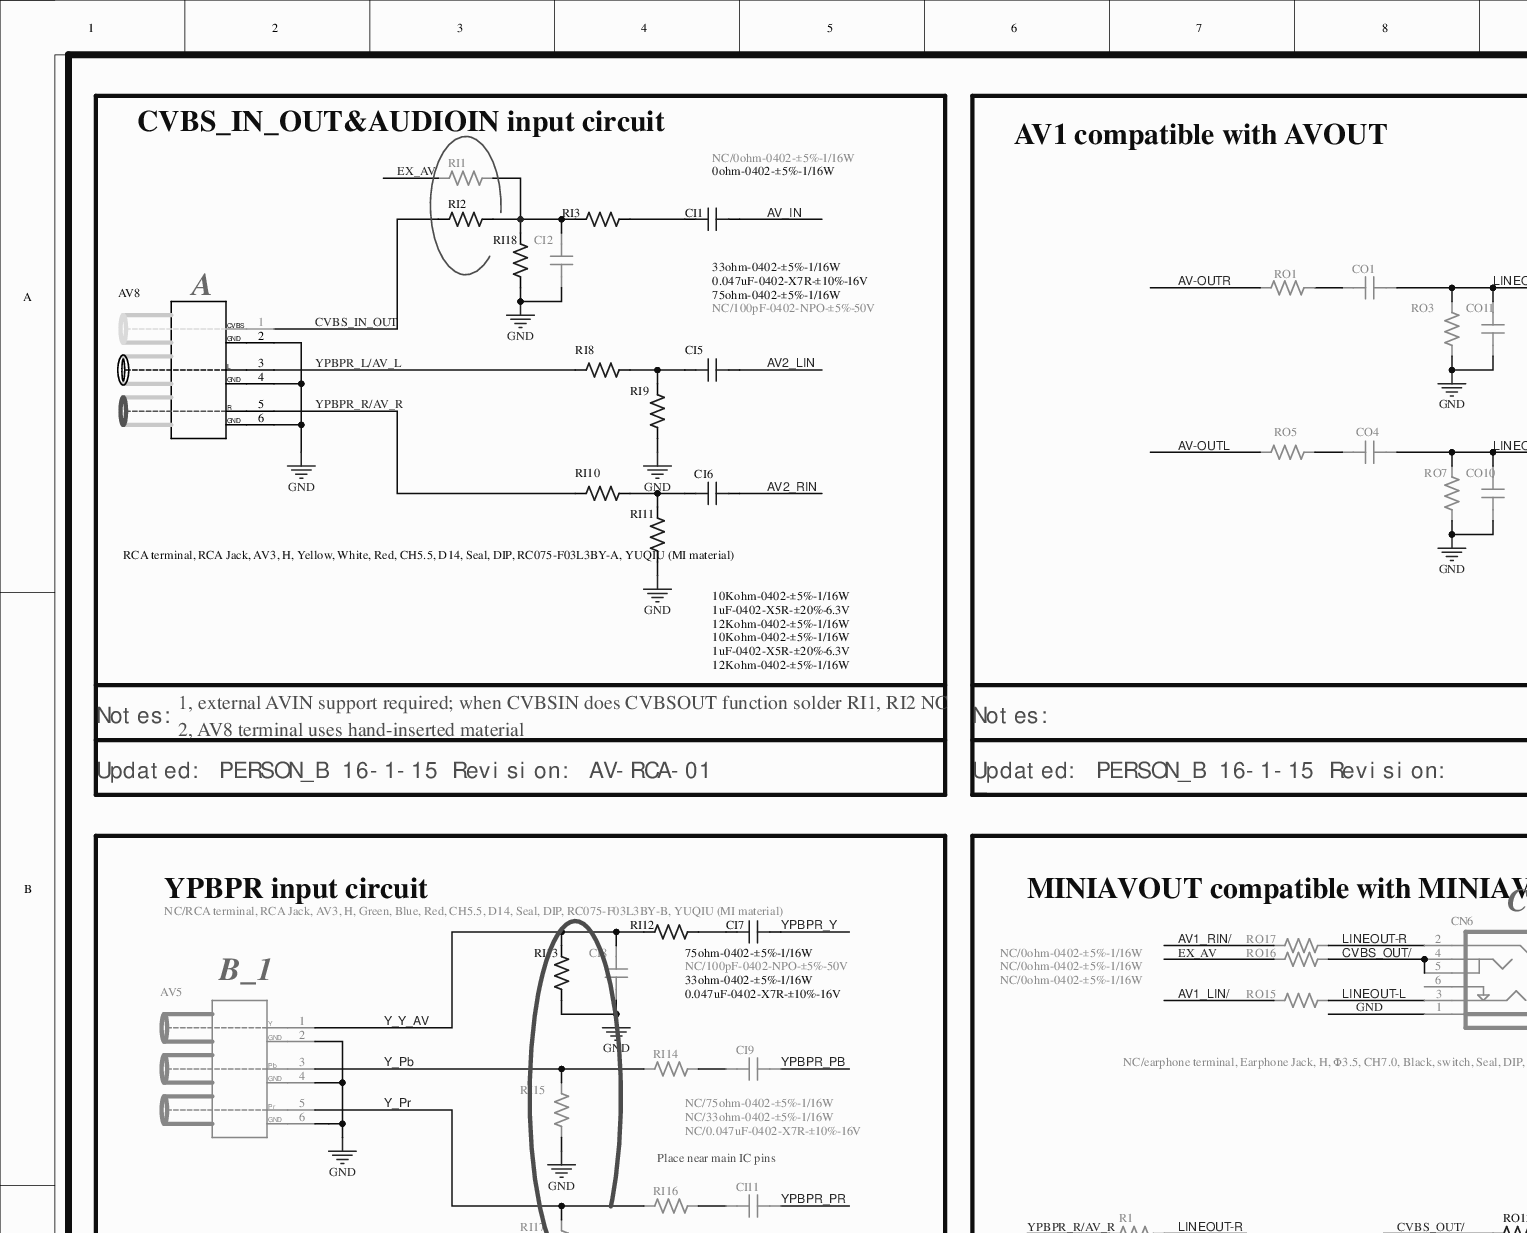
[diagram p0: MISC84277-9.SchDoc, top left]
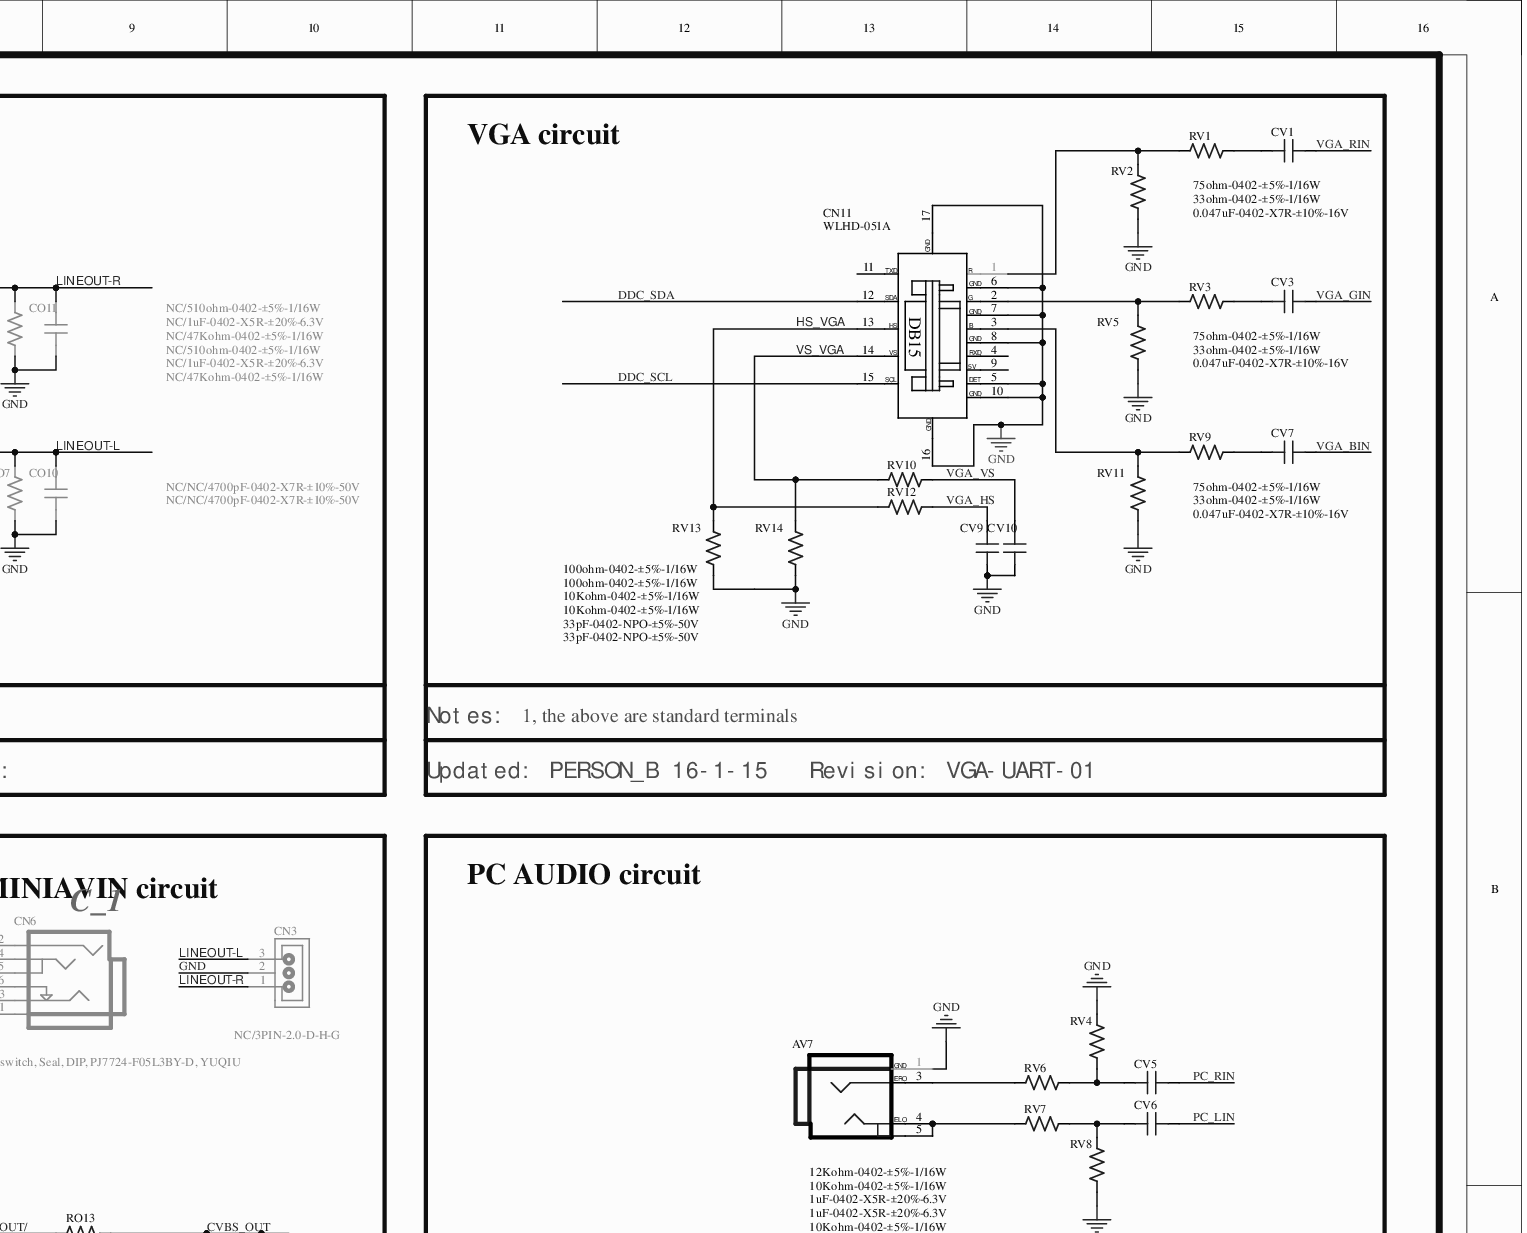
[diagram p1: MISC84277-9.SchDoc, top right]
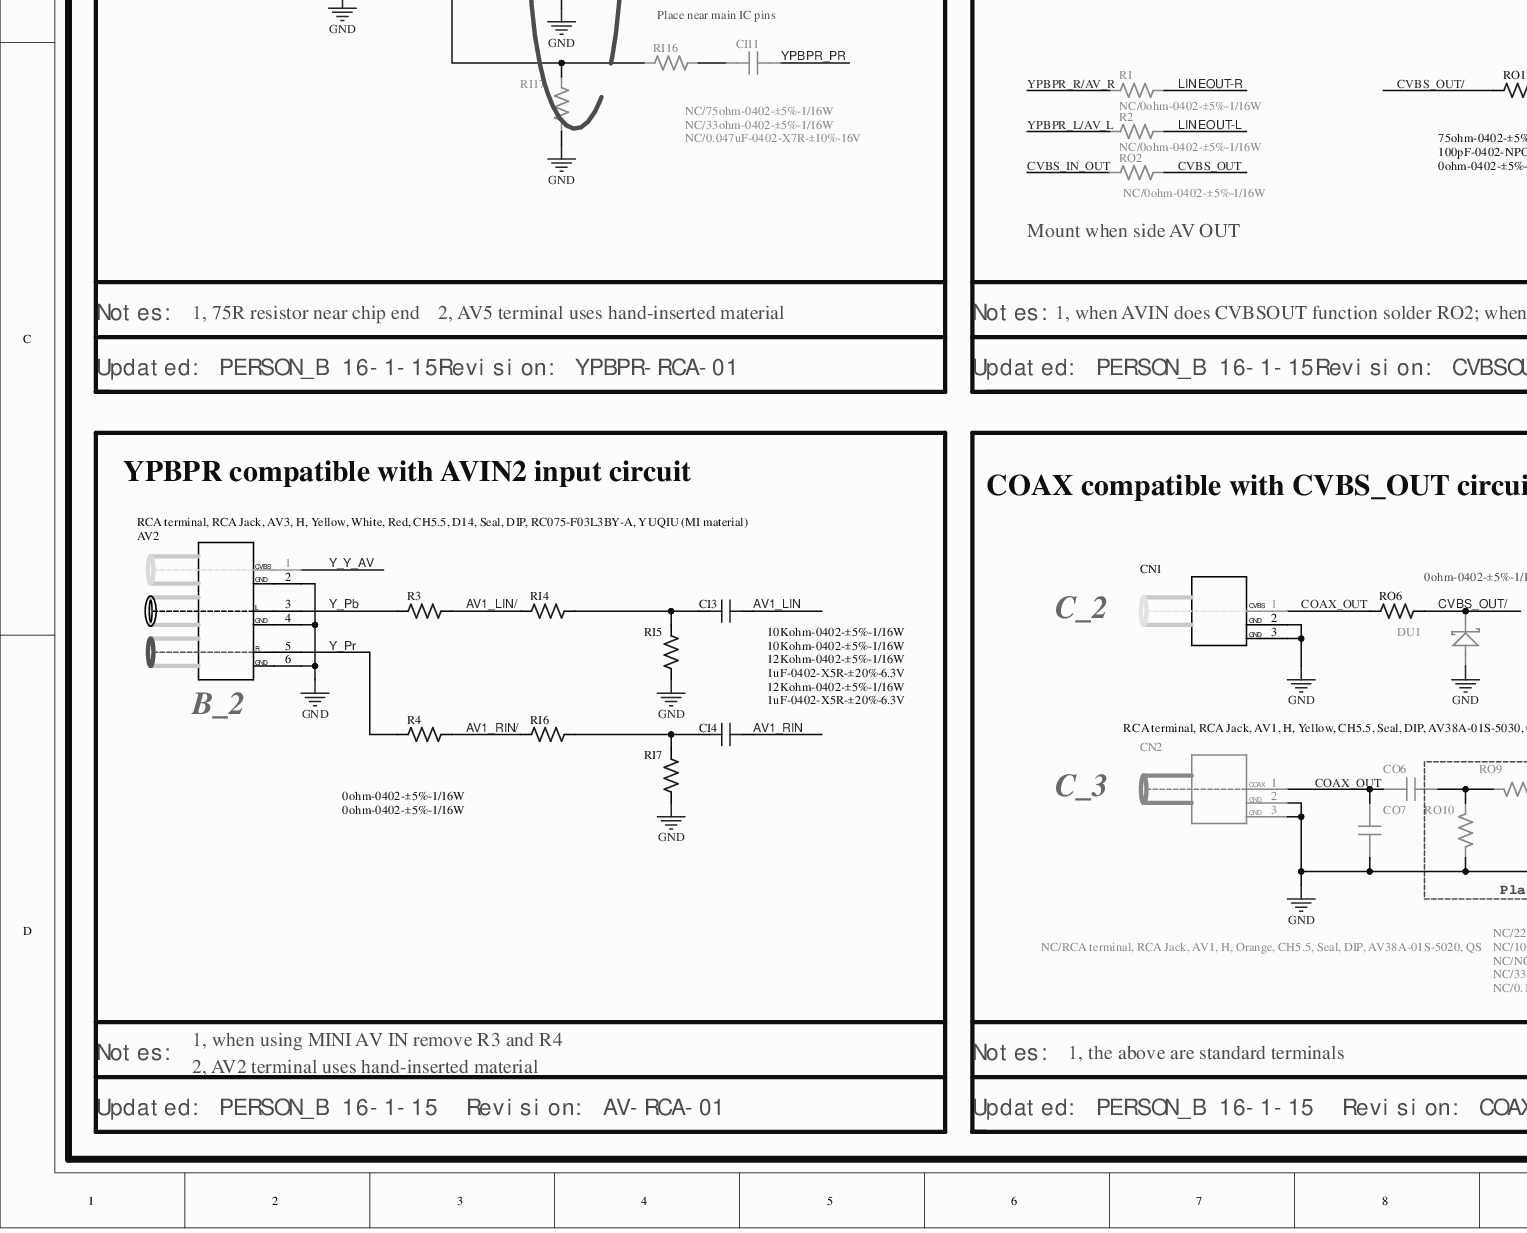
[diagram p2: MISC84277-9.SchDoc, bottom left]
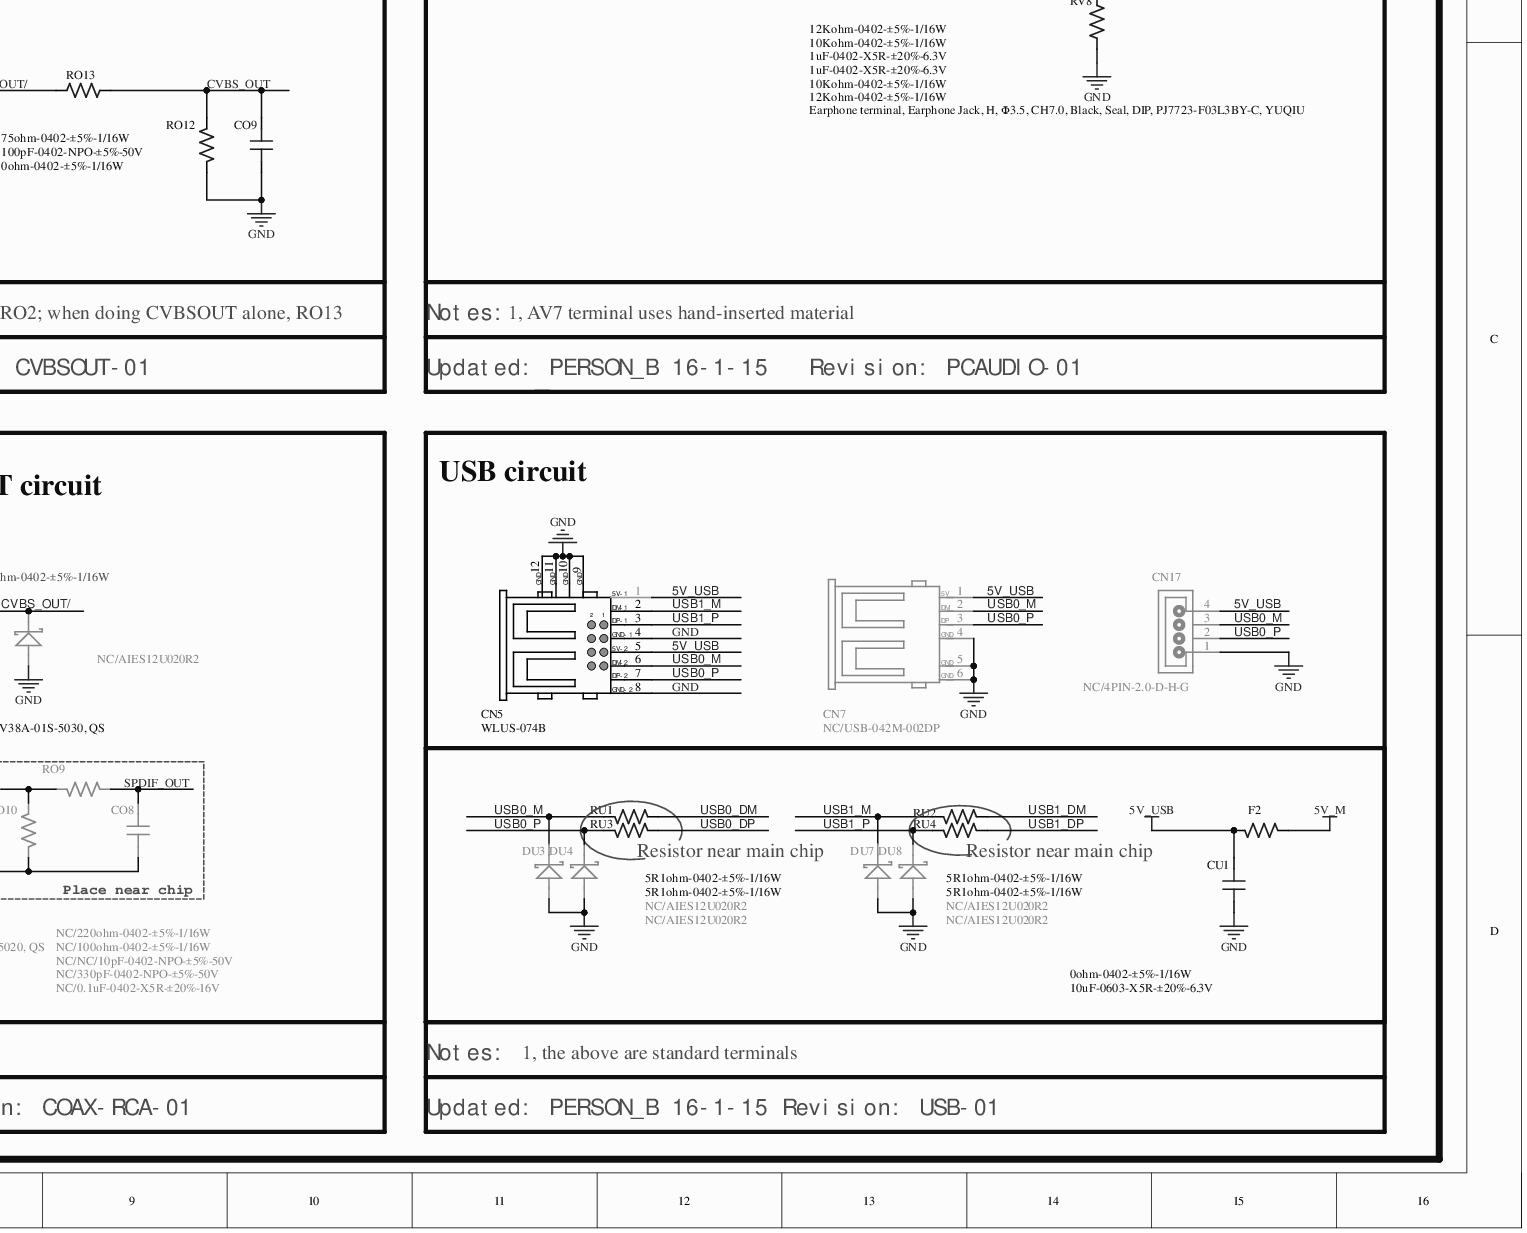
[diagram p3: MISC84277-9.SchDoc, bottom right]
# Altium project MISC84277-14.PrjPCB (part 8 of 10)

## Sheet MISC84277-9.SchDoc
size 548 x 439 mm

### Parts
AV2  RCA terminal, RCA Jack, AV3, H, Yellow, White, Red, CH5.5, D14, Seal, DIP, RC075-F03L3BY-A, YUQIU (MI material)  [AV3-H14-15]
AV5  NC/RCA terminal, RCA Jack, AV3, H, Green, Blue, Red, CH5.5, D14, Seal, DIP, RC075-F03L3BY-B, YUQIU (MI material)  [AV3-H14-15]
AV7  Earphone terminal, Earphone Jack, H, Φ3.5, CH7.0, Black, Seal, DIP, PJ7723-F03L3BY-C, YUQIU  [PHONE-HD-41]
AV8  RCA terminal, RCA Jack, AV3, H, Yellow, White, Red, CH5.5, D14, Seal, DIP, RC075-F03L3BY-A, YUQIU (MI material)  [AV3-H14-15]
CI1  0.047uF-0402-X7R-±10%-16V  [C0402]
CI2  NC/100pF-0402-NPO-±5%-50V  [C0402]
CI3  1uF-0402-X5R-±20%-6.3V  [C0402]
CI4  1uF-0402-X5R-±20%-6.3V  [C0402]
CI5  1uF-0402-X5R-±20%-6.3V  [C0402]
CI6  1uF-0402-X5R-±20%-6.3V  [C0402]
CI7  0.047uF-0402-X7R-±10%-16V  [C0402]
CI8  NC/100pF-0402-NPO-±5%-50V  [C0402]
CI9  NC/0.047uF-0402-X7R-±10%-16V  [C0402]
CI11  NC/0.047uF-0402-X7R-±10%-16V  [C0402]
CN1  RCA terminal, RCA Jack, AV1, H, Yellow, CH5.5, Seal, DIP, AV38A-01S-5030, QS  [AV1-H-4]
CN2  NC/RCA terminal, RCA Jack, AV1, H, Orange, CH5.5, Seal, DIP, AV38A-01S-5020, QS  [AV1-H-4]
CN3  NC/3PIN-2.0-D-H-G  [SIP3/2.0D-1]
CN5  WLUS-074B  [USB2-HD-1]
CN6  NC/earphone terminal, Earphone Jack, H, Φ3.5, CH7.0, Black, switch, Seal, DIP, PJ7724-F05L3BY-D, YUQIU  [PHONE-HD-42]
CN7  NC/USB-042M-002DP  [USB1-HD-2]
CN11  WLHD-051A  [DB15-HF-1]
CN17  NC/4PIN-2.0-D-H-G  [SIP4/2.0D-1]
CO1  NC/1uF-0402-X5R-±20%-6.3V  [C0402]
CO4  NC/1uF-0402-X5R-±20%-6.3V  [C0402]
CO6  NC/0.1uF-0402-X5R-±20%-16V  [C0402]
CO7  NC/330pF-0402-NPO-±5%-50V  [C0402]
CO8  NC/NC/10pF-0402-NPO-±5%-50V  [C0402]
CO9  100pF-0402-NPO-±5%-50V  [C0402]
CO10  NC/NC/4700pF-0402-X7R-±10%-50V  [C0402]
CO11  NC/NC/4700pF-0402-X7R-±10%-50V  [C0402]
CU1  10uF-0603-X5R-±20%-6.3V  [C0603]
CV1  0.047uF-0402-X7R-±10%-16V  [C0402]
CV3  0.047uF-0402-X7R-±10%-16V  [C0402]
CV5  1uF-0402-X5R-±20%-6.3V  [C0402]
CV6  1uF-0402-X5R-±20%-6.3V  [C0402]
CV7  0.047uF-0402-X7R-±10%-16V  [C0402]
CV9  33pF-0402-NPO-±5%-50V  [C0402]
CV10  33pF-0402-NPO-±5%-50V  [C0402]
DU1  NC/AIES12U020R2  [DIODE-S0402]
DU3  NC/AIES12U020R2  [DIODE-S0402]
DU4  NC/AIES12U020R2  [DIODE-S0402]
DU7  NC/AIES12U020R2  [DIODE-S0402]
DU8  NC/AIES12U020R2  [DIODE-S0402]
F2  0ohm-0402-±5%-1/16W  [R0402]
R1  NC/0ohm-0402-±5%-1/16W  [R0402]
R2  NC/0ohm-0402-±5%-1/16W  [R0402]
R3  0ohm-0402-±5%-1/16W  [R0402]
R4  0ohm-0402-±5%-1/16W  [R0402]
RI1  NC/0ohm-0402-±5%-1/16W  [R0402]
RI2  0ohm-0402-±5%-1/16W  [R0402]
RI3  33ohm-0402-±5%-1/16W  [R0402]
RI4  10Kohm-0402-±5%-1/16W  [R0402]
RI5  12Kohm-0402-±5%-1/16W  [R0402]
RI6  10Kohm-0402-±5%-1/16W  [R0402]
RI7  12Kohm-0402-±5%-1/16W  [R0402]
RI8  10Kohm-0402-±5%-1/16W  [R0402]
RI9  12Kohm-0402-±5%-1/16W  [R0402]
RI10  10Kohm-0402-±5%-1/16W  [R0402]
RI11  12Kohm-0402-±5%-1/16W  [R0402]
RI12  33ohm-0402-±5%-1/16W  [R0402]
RI13  75ohm-0402-±5%-1/16W  [R0402]
RI14  NC/33ohm-0402-±5%-1/16W  [R0402]
RI15  NC/75ohm-0402-±5%-1/16W  [R0402]
RI16  NC/33ohm-0402-±5%-1/16W  [R0402]
RI17  NC/75ohm-0402-±5%-1/16W  [R0402]
RI18  75ohm-0402-±5%-1/16W  [R0402]
RO1  NC/510ohm-0402-±5%-1/16W  [R0402]
RO2  NC/0ohm-0402-±5%-1/16W  [R0402]
RO3  NC/47Kohm-0402-±5%-1/16W  [R0402]
RO5  NC/510ohm-0402-±5%-1/16W  [R0402]
RO6  0ohm-0402-±5%-1/16W  [R0402]
RO7  NC/47Kohm-0402-±5%-1/16W  [R0402]
RO9  NC/220ohm-0402-±5%-1/16W  [R0402]
RO10  NC/100ohm-0402-±5%-1/16W  [R0402]
RO12  75ohm-0402-±5%-1/16W  [R0402]
RO13  0ohm-0402-±5%-1/16W  [R0402]
RO15  NC/0ohm-0402-±5%-1/16W  [R0402]
RO16  NC/0ohm-0402-±5%-1/16W  [R0402]
RO17  NC/0ohm-0402-±5%-1/16W  [R0402]
RU1  5R1ohm-0402-±5%-1/16W  [R0402]
RU2  5R1ohm-0402-±5%-1/16W  [R0402]
RU3  5R1ohm-0402-±5%-1/16W  [R0402]
RU4  5R1ohm-0402-±5%-1/16W  [R0402]
RV1  33ohm-0402-±5%-1/16W  [R0402]
RV2  75ohm-0402-±5%-1/16W  [R0402]
RV3  33ohm-0402-±5%-1/16W  [R0402]
RV4  12Kohm-0402-±5%-1/16W  [R0402]
RV5  75ohm-0402-±5%-1/16W  [R0402]
RV6  10Kohm-0402-±5%-1/16W  [R0402]
RV7  10Kohm-0402-±5%-1/16W  [R0402]
RV8  12Kohm-0402-±5%-1/16W  [R0402]
RV9  33ohm-0402-±5%-1/16W  [R0402]
RV10  100ohm-0402-±5%-1/16W  [R0402]
RV11  75ohm-0402-±5%-1/16W  [R0402]
RV12  100ohm-0402-±5%-1/16W  [R0402]
RV13  10Kohm-0402-±5%-1/16W  [R0402]
RV14  10Kohm-0402-±5%-1/16W  [R0402]

### Blocks framed on the sheet
A: AV8 CI1 CI2 CI5 CI6 RI1-RI3 RI8-RI11 RI18
VGA circuit: CN11 CV1 CV3 CV7 CV9 CV10 RV1-RV3 RV5 RV9-RV14
B_2: AV2 CI3 CI4 R3 R4 RI4-RI7
USB circuit: CN5 CN7 CN17 CU1 DU3 DU4 DU7 DU8 F2 RU1-RU4
Place near chip: CO8 RO9 RO10

### Nets
5V_M: F2.1
5V_USB: CN5.1 CN5.5 CN7.1 CN17.4 CU1.2 F2.2
GND: AV2.2(GND) AV2.4 AV2.6 AV5.2(CVBS) AV5.4(Rin) AV5.6(Lin) AV7.1 AV8.2(GND) AV8.4 AV8.6 CI2.2 CI8.2 CN1.2(GND) CN1.3(GND) CN2.2(GND) CN2.3(GND) CN3.2 CN5.4 CN5.8 CN5.9 CN5.10 CN5.11 CN5.12 CN6.1 CN7.4 CN7.5 CN7.6 CN11.5 CN11.6(GND) CN11.7(GND) CN11.8(GND) CN11.10(GND) CN11.16(Shell) CN11.17(Shell) CN17.1 CO7.2 CO8.2 CO9.1 CO10.1 CO11.1 CU1.1 CV9.2 CV10.2 DU1.A DU3.A DU4.A DU7.A DU8.A RI5.1 RI7.2 RI9.1 RI11.2 RI13.1 RI15.1 RI17.1 RI18.1 RO3.1 RO7.1 RO10.2 RO12.2 RV2.1 RV4.1 RV5.1 RV8.2 RV11.1 RV13.2 RV14.2
AV1_LIN: CI3.1
AV1_LIN/: R3.2 RI4.2 RO15.1
AV1_RIN: CI4.1
AV1_RIN/: R4.2 RI6.2 RO17.1
AV2_LIN: CI5.1
AV2_RIN: CI6.1
AV-OUTL: RO5.1
AV-OUTR: RO1.1
AV_IN: CI1.1
COAX_OUT: CN1.1(CVBS) CN2.1(CVBS) CO6.1 CO7.1 RO6.1
CVBS_IN_OUT: AV8.1(R) RI2.1 RO2.1
CVBS_OUT: CO9.2 RO2.2 RO12.1 RO13.2
CVBS_OUT/: CN6.4 CN6.5 DU1.K RO6.2 RO13.1 RO16.2
DDC_SCL: CN11.15(SCL)
DDC_SDA: CN11.12(SDA)
EX_AV: RI1.1 RO16.1
HS_VGA: CN11.13(HS) RV12.1 RV13.1
LINEOUT-L: CN3.3 CN6.3 CO4.1 CO10.2 R2.2 RO7.2 RO15.2
LINEOUT-R: CN3.1 CN6.2 CO1.1 CO11.2 R1.2 RO3.2 RO17.2
PC_LIN: CV6.2
PC_RIN: CV5.2
SPDIF_OUT: CO8.1 RO9.1
USB0_DM: RU1.1
USB0_DP: RU3.1
USB0_M: CN5.6 CN7.2 CN17.3 DU3.K RU1.2
USB0_P: CN5.7 CN7.3 CN17.2 DU4.K RU3.2
USB1_DM: RU2.1
USB1_DP: RU4.1
USB1_M: CN5.2 DU7.K RU2.2
USB1_P: CN5.3 DU8.K RU4.2
VGA_BIN: CV7.1
VGA_GIN: CV3.1
VGA_HS: CV9.1 RV12.2
VGA_RIN: CV1.1
VGA_VS: CV10.1 RV10.2
VS_VGA: CN11.14(VS) RV10.1 RV14.1
Y_Pb: AV2.3 AV5.3(GND) R3.1 RI14.2 RI15.2
Y_Pr: AV2.5 AV5.5(GND) R4.1 RI16.2 RI17.2
Y_Y_AV: AV2.1(R) AV5.1(GND) CI8.1 RI12.1 RI13.2
YPBPR_L/AV_L: AV8.3 R2.1 RI8.2
YPBPR_PB: CI9.1
YPBPR_PR: CI11.1
YPBPR_R/AV_R: AV8.5 R1.1 RI10.2
YPBPR_Y: CI7.1
NetAV7_3: AV7.3 RV6.2
NetAV7_4: AV7.4 AV7.5 RV7.2
NetCI1_2: CI1.2 RI3.1
NetCI2_1: CI2.1 RI1.2 RI2.2 RI3.2 RI18.2
NetCI3_2: CI3.2 RI4.1 RI5.2
NetCI4_2: CI4.2 RI6.1 RI7.1
NetCI5_2: CI5.2 RI8.1 RI9.2
NetCI6_2: CI6.2 RI10.1 RI11.1
NetCI7_2: CI7.2 RI12.2
NetCI9_2: CI9.2 RI14.1
NetCI11_2: CI11.2 RI16.1
NetCN11_1: CN11.1(R) RV1.2 RV2.2
NetCN11_2: CN11.2(G) RV3.2 RV5.2
NetCN11_3: CN11.3(B) RV9.2 RV11.2
NetCO1_2: CO1.2 RO1.2
NetCO4_2: CO4.2 RO5.2
NetCO6_2: CO6.2 RO9.2 RO10.1
NetCV1_2: CV1.2 RV1.1
NetCV3_2: CV3.2 RV3.1
NetCV5_1: CV5.1 RV4.2 RV6.1
NetCV6_1: CV6.1 RV7.1 RV8.1
NetCV7_2: CV7.2 RV9.1

Not connected (* = marked no-connect by the designer): CN6 6*; CN11 4(NC)* 9(NC)* 11(NC)*

### Notes on the sheet
- (near RI1) CVBS_IN_OUT&AUDIOIN input circuit
- AV1 compatible with AVOUT
- Notes:
- 1, external AVIN support required; when CVBSIN does CVBSOUT function solder RI1, RI2 NC
- 2, AV8 terminal uses hand-inserted material
- 1, the above are standard terminals
- Updated: PERSON_B 16-1-15
- Revision: AV-RCA-01
- Revision:
- Revision: VGA-UART-01
- PC AUDIO circuit
- YPBPR input circuit
- MINIAVOUT compatible with MINIAVIN circuit
- C_1
- (near AV5) B_1
- Place near main IC pins
- (near RO2) Mount when side AV OUT
- 1, 75R resistor near chip end
- 2, AV5 terminal uses hand-inserted material
- 1, when AVIN does CVBSOUT function solder RO2; when doing CVBSOUT alone, RO13
- 1, AV7 terminal uses hand-inserted material
- Revision: YPBPR-RCA-01
- Revision: CVBSOUT-01
- Revision: PCAUDIO-01
- YPBPR compatible with AVIN2 input circuit
- COAX compatible with CVBS_OUT circuit
- C_2
- C_3
- Resistor near main chip
- (near RU4) Resistor near main chip
- 1, when using MINI AV IN remove R3 and R4
- 2, AV2 terminal uses hand-inserted material
- Revision: COAX-RCA-01
- Revision: USB-01

### Library data of the parts
AV2 AV8 = RCA端子,RCA Jack,AV3,H,Yellow、White、Red,CH5.5,D14,Seal,DIP,RC075-F03L3BY-A,YUQIU-DLMI-AV: CN-AV-D14-#-#
AV5 = RCA端子,RCA Jack,AV3,H,Green、Blue、Red,CH5.5,D14,Seal,DIP,RC075-F03L3BY-B,YUQIU-DLMI-YPbPr: CN-YPbPr-D14-#-#
AV7 = 耳机端子,Earphone  Jack,H,Φ3.5,CH7.0,Black,Seal,SMD,PJ7723-F03L3BE-C,YUQIU-DLMI: CN-headphone
CI1 CI7 CI9 CI11 CV1 CV3 CV7 = 0.047uF-0402-X7R-±10%-16V-D
CI2 CO9 = 100pF-0402-NPO-±5%-50V-D
CI3-CI6 CO6 CV5 CV6 = 0.1uF-0402-Y5V-+80%-20%-16V-D
CI8 CO8 = 10pF-0402-NPO-±5%-50V-D
CN1 = RCA端子,RCA Jack,AV1,H,Yellow,CH5.5,Seal,DIP,AV38A-01S-5030,QS-DLMI
CN2 = RCA端子,RCA Jack,AV1,H,Orange,CH5.5,Seal,DIP,AV38A-01S-5020,QS-DLMI
CN3 = 3PIN-2.0-D-H-G-DHMI
CN5 = USB-A/F-90°-DLMI-USB: CN-USB-double-deck-#-#
CN6 = 耳机端子,Earphone  Jack,H,Φ3.5,CH7.0,Black,switch,Seal,SMD,PJ7724-F05L3BE-D,YUQIU-DLMI-headphone: CN-headphone-#-#-#
CN7 = USB-2035A01-DHMI-USB: CN-USB-#-#-#
CN11 = WLHD-051A-DLMI-DB15: CN-DB15-horizontal-#-#-#
CN17 = 4PIN-2.0-D-H-G-DHMI
CO1 CO4 = 1uF-0402-X5R-±20%-6.3V-D
CO7 = 330pF-0402-X7R-±10%-50V-D
CO10 CO11 = 4700pF-0402-X7R-±10%-50V-D
CU1 = 10uF-0603-X5R-±20%-6.3V-D
CV9 CV10 = 33pF-0402-NPO-±5%-50V-D
DU1 DU3 DU4 DU7 DU8 = AIES12U020R2-D
F2 RU1-RU4 = 5R1ohm-0402-±5%-1/16W-D
R1-R4 RI1 RI2 RO2 RO6 RO13 RO15-RO17 = 0ohm-0402-±5%-1/16W-D
RI3 = 150ohm-0402-±5%-1/16W-D
RI4 RI6 RI8 RI10 RV6 RV7 RV13 RV14 = 10Kohm-0402-±5%-1/16W-D
RI5 RI7 RI9 RI11 RV4 RV8 = 12Kohm-0402-±5%-1/16W-D
RI12 RI14 RI16 RV1 RV3 RV9 = 33ohm-0402-±5%-1/16W-D
RI13 RI15 RI17 RI18 RO12 RV2 RV5 RV11 = 75ohm-0402-±5%-1/16W-D
RO1 RO5 = 510ohm-0402-±5%-1/16W-D
RO3 RO7 = 47Kohm-0402-±5%-1/16W-D
RO9 = 220ohm-0402-±5%-1/16W-D
RO10 RV10 RV12 = 100ohm-0402-±5%-1/16W-D